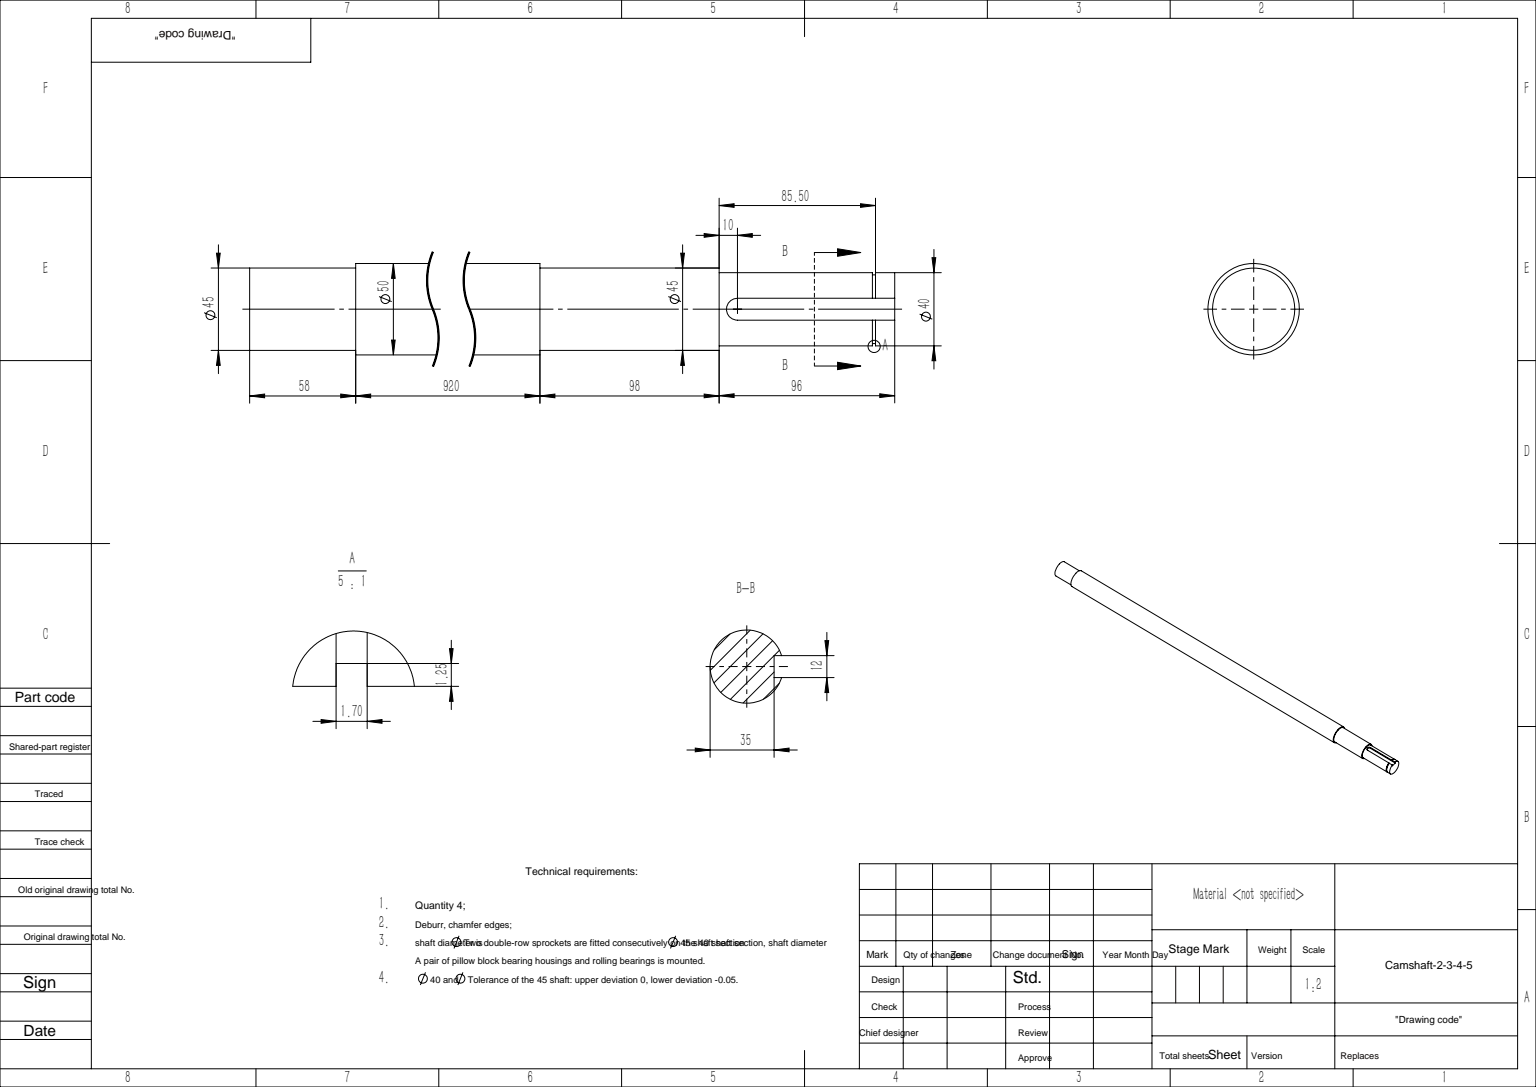
SolidWorks part; units mm, degrees
ref_plane "前视基准面" through (0, 0, 0) normal (0, 0, 1) x (1, 0, 0)
ref_plane "上视基准面" through (0, 0, 0) normal (0, 1, 0) x (1, 0, 0)
ref_plane "右视基准面" through (0, 0, 0) normal (1, 0, 0) x (0, 0, -1)
sketch "草图1" plane through (0, 0, 0) normal (0, 0, 1) x (1, 0, 0)
  line L0 (0, 0) -> (0, 22.5)
  line L1 (0, 22.5) -> (58, 22.5)
  line L2 (58, 22.5) -> (58, 25)
  line L3 (58, 25) -> (978, 25)
  line L4 (978, 25) -> (978, 22.5)
  line L5 (978, 22.5) -> (1076, 22.5)
  line L6 (1076, 22.5) -> (1076, 20)
  line L7 (1076, 20) -> (1172, 20)
  line L8 (1172, 20) -> (1172, 0)
  line L9 (1172, 0) -> (0, 0)
  dimension "D1" = 58
  dimension "D2" = 920
  dimension "D3" = 98
  dimension "D4" = 96
  dimension "D5" = 25
  dimension "D6" = 22.5
  dimension "D7" = 22.5
  dimension "D8" = 20
revolve "旋转1" add sketch "草图1" angle 360 about L9
ref_plane "基准面1" through (0, 20, 0) normal (0, 1, 0) x (1, 0, 0)
sketch "草图2" plane through (0, 20, 0) normal (0, 1, 0) x (1, 0, 0)
  line L0 (1076, 0) -> (1172, 0) construction
  line L3 (1076, -22.5) -> (1076, 22.5) construction
  line L4 (1172, -20) -> (1172, 20) construction
  line L5 (1076, -20) -> (1076, 20) construction
  line L6 (1086, 6) -> (1182, 6)
  line L7 (1086, -6) -> (1182, -6)
  line L9 (1182, 6) -> (1182, -6)
  arc A0 (1086, 6) -> (1086, -6) centre (1086, 0) ccw
  dimension "D1" = 12
  dimension "D3" = 10
  dimension "D2" = 10
extrude "切除-拉伸1" cut sketch "草图2" against normal blind 5
ref_plane "基准面2" through (1161.5, 0, 0) normal (1, 0, 0) x (0, 0, -1)
sketch "草图3" plane through (1161.5, 0, 0) normal (1, 0, 0) x (0, 0, -1)
  circle A0 centre (0, 0) radius 18.75
  circle A2 centre (0, 0) radius 20
  circle A3 centre (0, 0) radius 20 construction
  dimension "D2" = 37.5
extrude "切除-拉伸2" cut sketch "草图3" against normal blind 1.7
